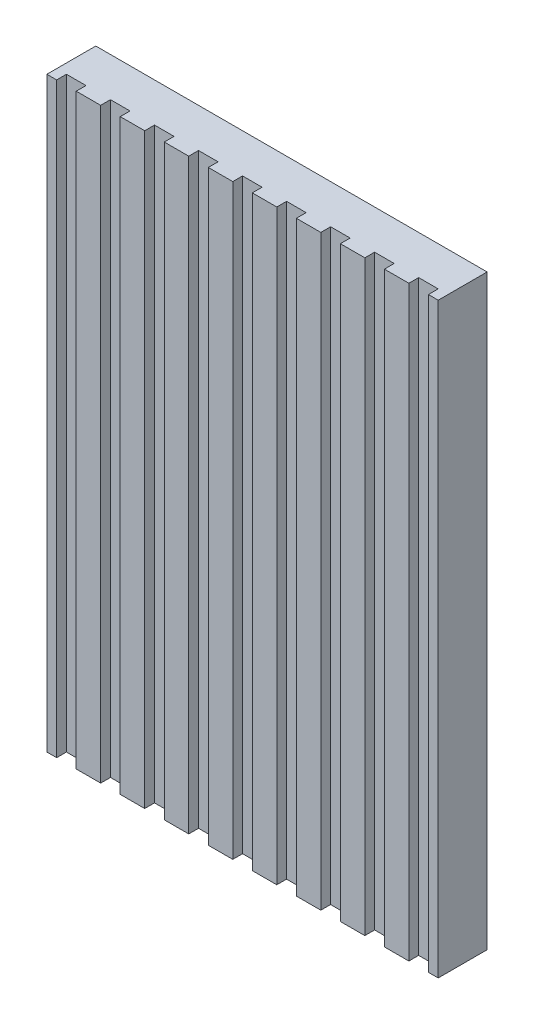
SolidWorks part; units mm, degrees
ref_plane "Front Plane" through (0, 0, 0) normal (0, 0, 1) x (1, 0, 0)
ref_plane "Top Plane" through (0, 0, 0) normal (0, 1, 0) x (1, 0, 0)
ref_plane "Right Plane" through (0, 0, 0) normal (1, 0, 0) x (0, 0, -1)
sketch "Sketch1" plane through (0, 0, 0) normal (0, 0, 1) x (1, 0, 0)
  line L1 (-400, 600) -> (400, 600)
  line L2 (-400, 600) -> (-400, -600)
  line L3 (-400, -600) -> (400, -600)
  line L4 (400, 600) -> (400, -600)
  line L5 (-400, 600) -> (400, -600) construction
  line L6 (-400, -600) -> (400, 600) construction
  point P0 (0, 0)
  dimension "D1" = 800
  dimension "D2" = 1200
extrude "Boss-Extrude1" add sketch "Sketch1" along normal blind 100
sketch "Sketch2" plane through (0, -600, 0) normal (0, -1, 0) x (1, 0, 0)
  line L0 (-400, 100) -> (400, 100) construction
  line L1 (-20, 120) -> (20, 120)
  line L2 (-20, 120) -> (-20, 80)
  line L3 (-20, 80) -> (20, 80)
  line L4 (20, 120) -> (20, 80)
  line L5 (-20, 120) -> (20, 80) construction
  line L6 (-20, 80) -> (20, 120) construction
  point P0 (0, 100)
  dimension "D1" = 20
  dimension "D2" = 40
extrude "Cut-Extrude1" cut sketch "Sketch2" against normal through all
pattern_linear "LPattern1" count 5 spacing 90 along (1, 0, 0) count 5 spacing 90 along (-1, 0, 0) seed only of "Cut-Extrude1"
